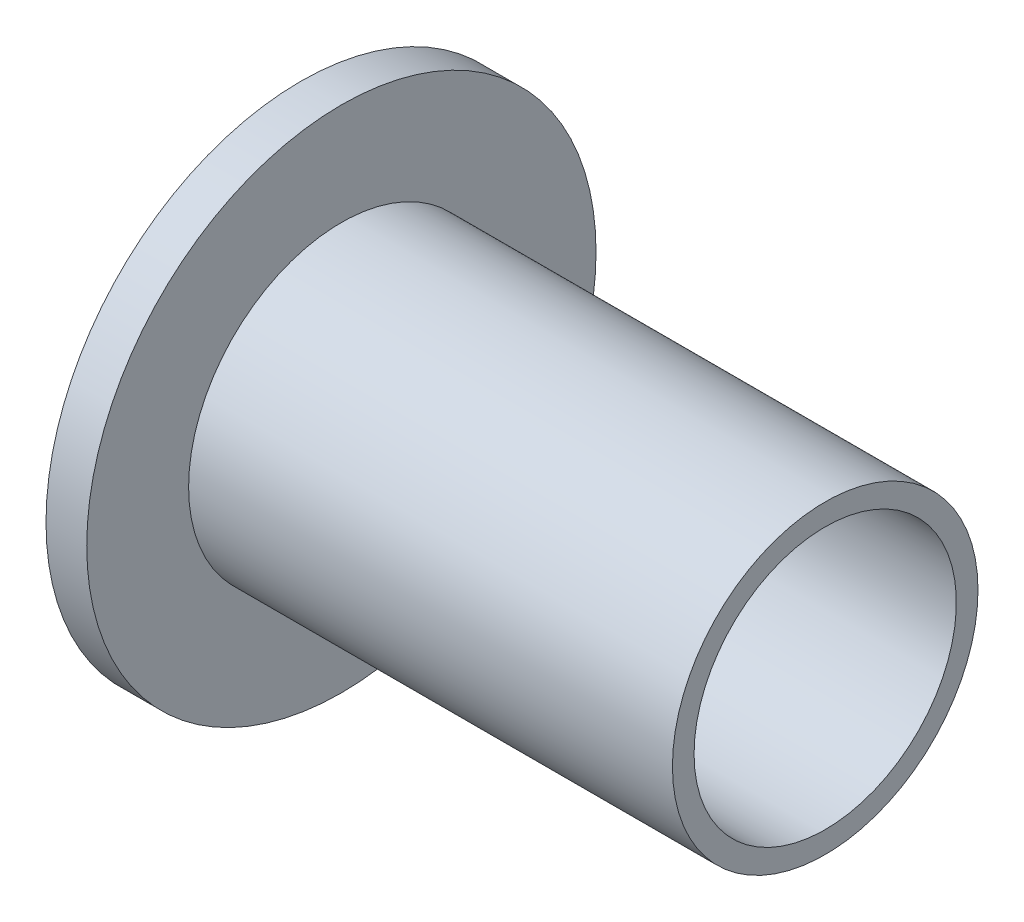
SolidWorks part; units mm, degrees
material "尼龙 101"
ref_plane "前视基准面" through (0, 0, 0) normal (0, 0, 1) x (1, 0, 0)
ref_plane "上视基准面" through (0, 0, 0) normal (0, 1, 0) x (1, 0, 0)
ref_plane "右视基准面" through (0, 0, 0) normal (1, 0, 0) x (0, 0, -1)
sketch "草图1" plane through (0, 0, 0) normal (0, 0, 1) x (1, 0, 0)
  line L0 (0, 0) -> (41.9789, 0) construction
  line L1 (0, 5.15) -> (0, 10)
  line L2 (0, 10) -> (1.6, 10)
  line L3 (1.6, 10) -> (1.6, 6)
  line L4 (1.6, 6) -> (20.6, 6)
  line L5 (20.6, 6) -> (20.6, 5.15)
  line L6 (20.6, 5.15) -> (0, 5.15)
  line L7 (0, 0) -> (0, 22.0485) construction
  dimension "D1" = 20
  dimension "D2" = 1.6
  dimension "D3" = 12
  dimension "D4" = 10.3
  dimension "D5" = 20.6
revolve "旋转1" add sketch "草图1" angle 360 about L0
